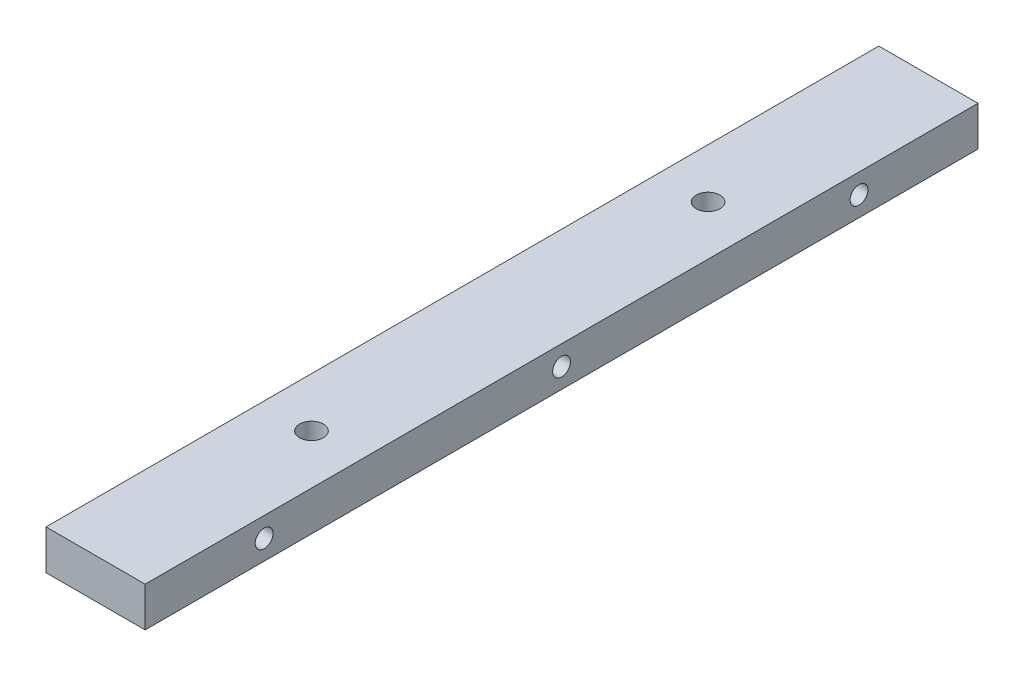
from build123d import *

# Parameters (mm, degrees)
SKETCH_1_W                = 210
SKETCH_1_H                = 10
EXTRUDE_1_DEPTH           = 12.5
HOLE_WIZARD_1_D           = 4.5
HOLE_WIZARD_1_CBORE_D     = 8
HOLE_WIZARD_1_CBORE_DEPTH = 5
SKETCH_5_R                = 3
CUT_EXTRUDE_1_DEPTH       = 29


with BuildPart() as part:
    # 草图1 → 凸台-拉伸1 (new, symmetric)
    with BuildSketch(Plane(origin=(0, 0, 0), x_dir=(0, 0, -1), z_dir=(1, 0, 0))):
        Rectangle(SKETCH_1_W, SKETCH_1_H)
    extrude(amount=EXTRUDE_1_DEPTH, both=True)

    # 打孔尺寸(%根据)开槽圆柱头螺钉的类型1 (through all)
    with Locations(Plane.ZY.offset(12.5)):
        with Locations((0, 0), (-75, 0), (75, 0)):
            CounterBoreHole(HOLE_WIZARD_1_D / 2, HOLE_WIZARD_1_CBORE_D / 2, HOLE_WIZARD_1_CBORE_DEPTH)

    # 草图5 → 切除-拉伸1 (cut)
    with BuildSketch(Plane.XZ.offset(5)):
        with Locations(Location((0, 50.563507408, 0), (0, 0, 270))):
            Circle(SKETCH_5_R)
        with Locations(Location((0, -49.436492592, 0), (0, 0, 270))):
            Circle(SKETCH_5_R)
    extrude(amount=-CUT_EXTRUDE_1_DEPTH, mode=Mode.SUBTRACT)


solid = part.part
